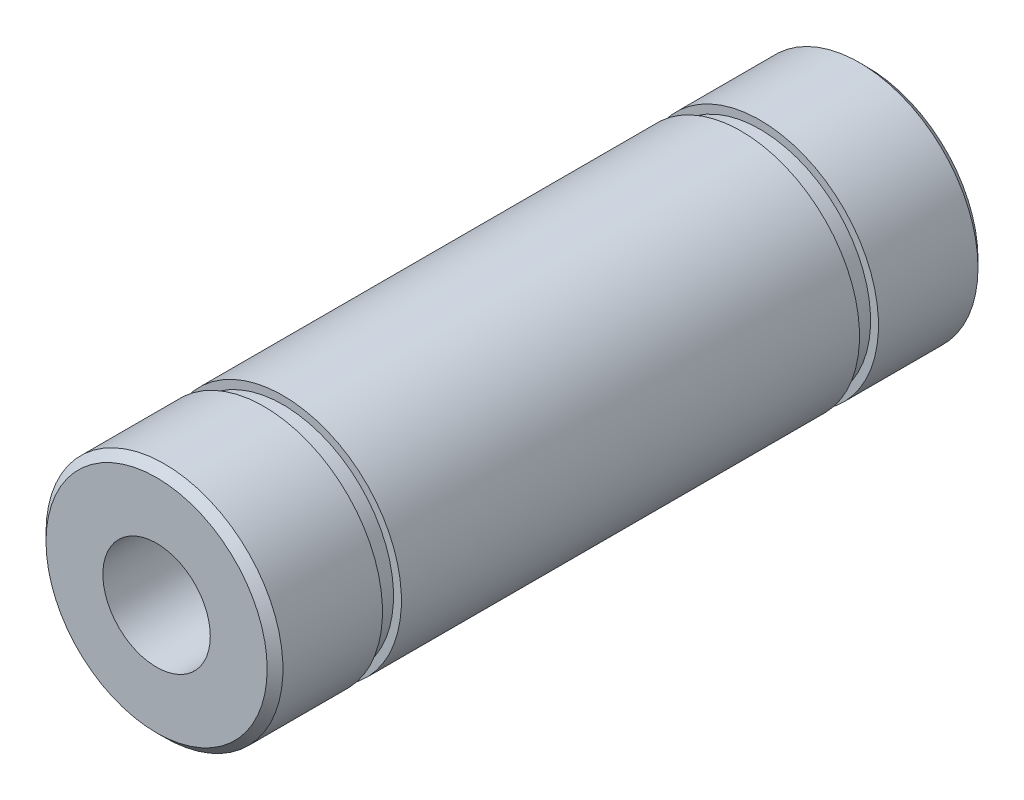
from build123d import *

# Parameters (mm, degrees)
SKETCH_1_R      = 7.5
EXTRUDE_1_DEPTH = 22.5
CHAMFER_1_SIZE  = 0.5
SKETCH_4_W      = 0.5
SKETCH_4_H      = 1.2


with BuildPart() as part:
    # 草图1 → 凸台-拉伸1 (new, symmetric)
    with BuildSketch(Plane.XY):
        with Locations(Location((0, 0, 0), (0, 0, 180))):
            Circle(SKETCH_1_R)
    extrude(amount=EXTRUDE_1_DEPTH, both=True)

    # 草图2 → M8 螺纹孔1 (revolve, cut)
    with BuildSketch(Plane(origin=(0, 0, 22.5), x_dir=(0, -1, 0), z_dir=(1, 0, 0))):
        Polygon((0, 0), (0, 22.042926105), (3.4, 20), (3.4, 0), align=None)
    hole_wizard_m8_1 = revolve(axis=Axis((0, 0, 28.85), (0, 0, -1)), mode=Mode.SUBTRACT)

    # 倒角1
    chamfer_1_edges = [part.edges().sort_by_distance(p)[0] for p in [
        (7.5, 0, -22.5),
        (7.5, 0, 22.5),
    ]]
    chamfer(chamfer_1_edges, length=CHAMFER_1_SIZE)

    # 镜向3: M8 螺纹孔1 across plane
    add(hole_wizard_m8_1.mirror(Plane.XY), mode=Mode.SUBTRACT)

    # 草图4 → 切除-旋转1 (revolve, cut)
    with BuildSketch(Plane(origin=(0, 0, 0), x_dir=(1, 0, 0), z_dir=(0, 1, 0)), mode=Mode.PRIVATE) as cut_revolve_1_sk:
        with Locations((7.25, 15.1)):
            Rectangle(SKETCH_4_W, SKETCH_4_H)
    cut_revolve_1 = revolve(cut_revolve_1_sk.sketch.rotate(Axis((0, 0, -24.688510649), (0, 0, 1)), 180), axis=Axis((0, 0, -24.688510649), (0, 0, 1)), mode=Mode.SUBTRACT)

    # 镜向5: 切除-旋转1 across plane
    add(cut_revolve_1.mirror(Plane.XY), mode=Mode.SUBTRACT)


solid = part.part
